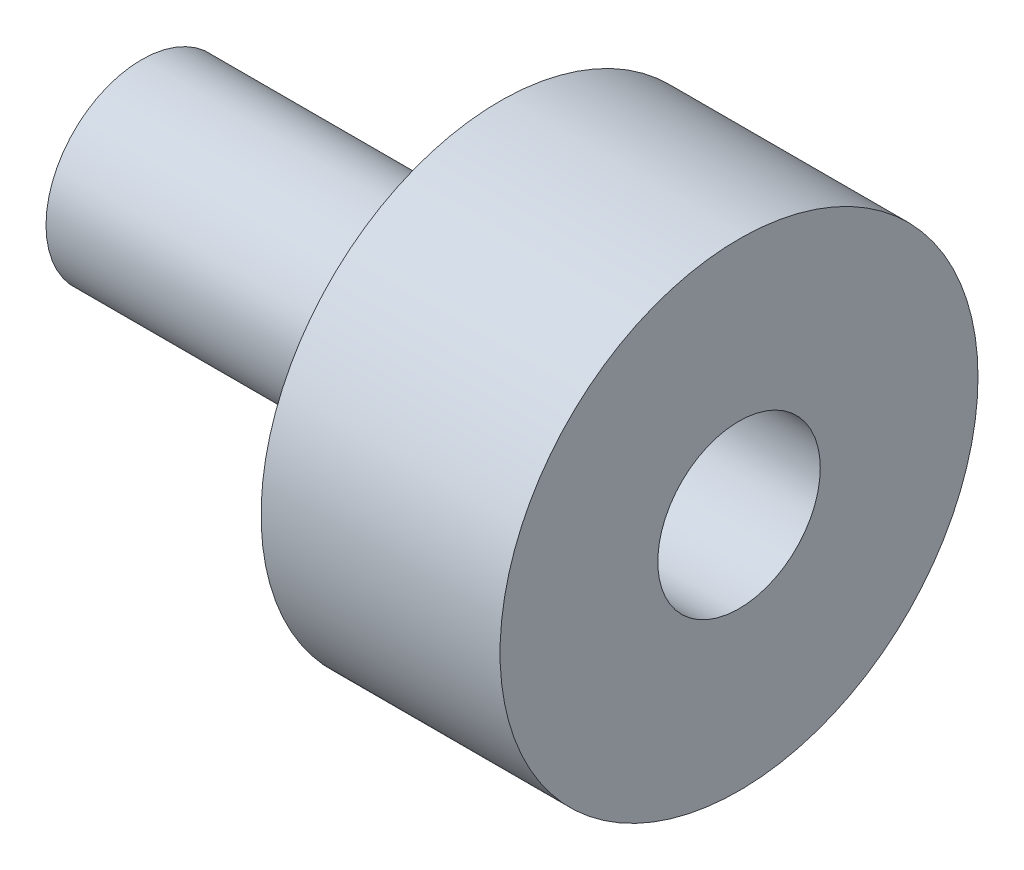
from build123d import *

# Parameters (mm, degrees)
SKETCH_1_R             = 10
EXTRUDE_1_DEPTH        = 10
SKETCH_2_R             = 4
EXTRUDE_2_DEPTH        = 15
HOLE_WIZARD_M8_1_D     = 6.8
HOLE_WIZARD_M8_1_DEPTH = 8
HOLE_WIZARD_M8_1_TIP   = 2.042926105


with BuildPart() as part:
    # 草图1 → 凸台-拉伸1 (new body)
    with BuildSketch(Plane(origin=(0, 0, 0), x_dir=(0, 0, -1), z_dir=(1, 0, 0))):
        Circle(SKETCH_1_R)
    extrude(amount=EXTRUDE_1_DEPTH)

    # 草图2 → 凸台-拉伸2 (add)
    with BuildSketch(Plane.ZY):
        Circle(SKETCH_2_R)
    extrude(amount=EXTRUDE_2_DEPTH)

    # M8 螺纹孔1
    with Locations(Plane(origin=(10, 0, 0), x_dir=(0, 0, -1), z_dir=(1, 0, 0))):
        with Locations((0, 0)):
            Hole(HOLE_WIZARD_M8_1_D / 2, depth=HOLE_WIZARD_M8_1_DEPTH)
            with Locations((0, 0, -(HOLE_WIZARD_M8_1_DEPTH + HOLE_WIZARD_M8_1_TIP / 2))):  # 118° drill point
                Cone(0, HOLE_WIZARD_M8_1_D / 2, HOLE_WIZARD_M8_1_TIP, mode=Mode.SUBTRACT)


solid = part.part
